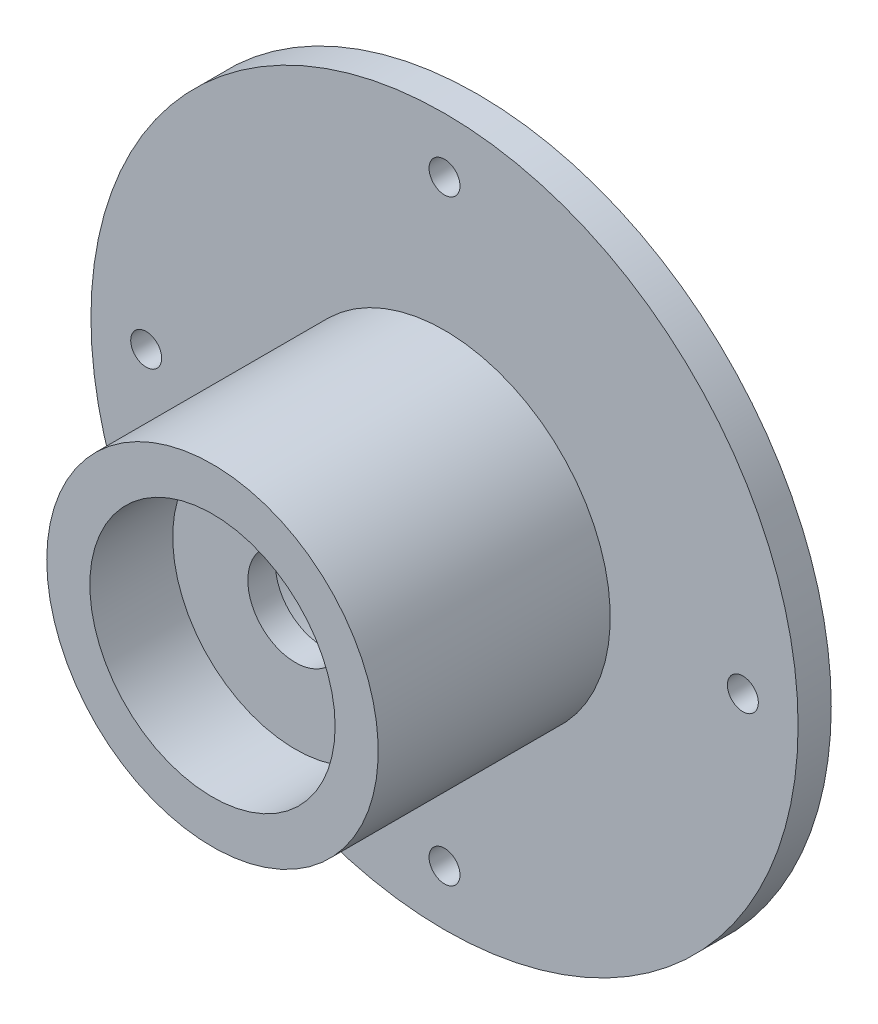
SolidWorks part; units mm, degrees
ref_plane "Front Plane" through (0, 0, 0) normal (0, 0, 1) x (1, 0, 0)
ref_plane "Top Plane" through (0, 0, 0) normal (0, 1, 0) x (1, 0, 0)
ref_plane "Right Plane" through (0, 0, 0) normal (1, 0, 0) x (0, 0, -1)
sketch "Sketch1" plane through (0, 0, 0) normal (0, 1, 0) x (1, 0, 0)
  line L0 (32, 0) -> (0, 0)
  line L1 (0, 0) -> (0, -3)
  line L2 (0, -3) -> (32, -3)
  line L3 (32, -3) -> (32, 0)
  line L4 (0, 0) -> (0, -3) construction
revolve "Revolve1" add sketch "Sketch1" angle 360 about L4
sketch "Sketch2" plane through (0, 0, 3) normal (0, 0, 1) x (1, 0, 0)
  circle A0 centre (0, 0) radius 15
extrude "Boss-Extrude1" add sketch "Sketch2" along normal blind 21
sketch "Sketch3" plane through (0, 0, 0) normal (0, 1, 0) x (1, 0, 0)
  line L0 (13, 0) -> (0, 0)
  line L1 (0, 0) -> (0, -24)
  line L2 (0, -24) -> (11.1, -24)
  line L3 (11.1, -24) -> (11.1, -16.5)
  line L4 (11.1, -16.5) -> (4.3, -16.5)
  line L5 (4.3, -16.5) -> (4.3, -14)
  line L6 (4.3, -14) -> (13, -14)
  line L7 (13, -14) -> (13, 0)
  line L8 (0, 0) -> (0, -24) construction
revolve "Cut-Revolve1" cut sketch "Sketch3" angle 360 about L8
hole_wizard "Ø2.8 (2.8) Diameter Hole1" positions "Sketch5" profile "Sketch4" hole size "Ø2.8" standard "ANSI Metric"
sketch "Sketch5" plane through (0, 0, 3) normal (0, 0, 1) x (1, 0, 0)
  point P0 (0, 27)
  point P1 (0, -27)
  point P2 (27, 0)
  point P3 (-27, 0)
sketch "Sketch4" plane through (0, 27, 3) normal (1, 0, 0) x (0, -1, 0)
  line L0 (0, 0) -> (0, 3)
  line L1 (0, 3) -> (1.4, 3)
  line L2 (1.4, 3) -> (1.4, 0)
  line L5 (1.4, 0) -> (0, 0)
  line L11 (0, -6.35) -> (0, 107.95) construction
  dimension "Thru Hole Dia." = 2.8
  dimension "Thru Hole Depth" = 3
fillet "Fillet1" [suppressed] radius 6
